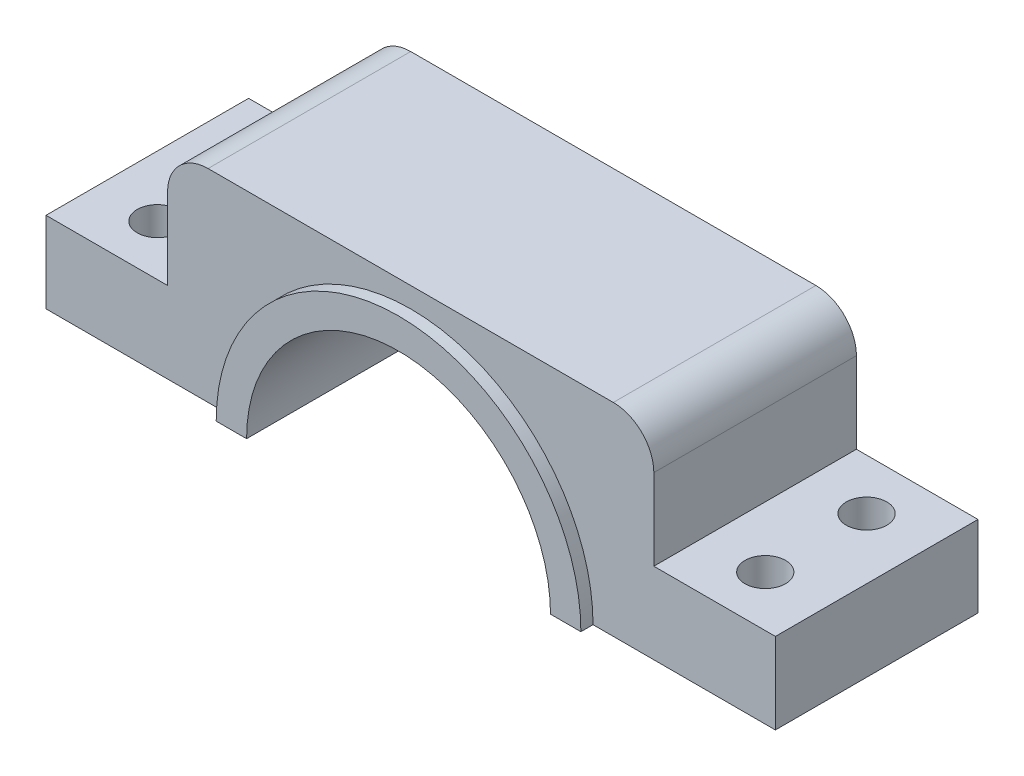
SolidWorks part; units mm, degrees
ref_plane "前视基准面" through (0, 0, 0) normal (0, 0, 1) x (1, 0, 0)
ref_plane "上视基准面" through (0, 0, 0) normal (0, 1, 0) x (1, 0, 0)
ref_plane "右视基准面" through (0, 0, 0) normal (1, 0, 0) x (0, 0, -1)
other "Configuration Table"
sketch "草图2" plane through (0, 0, 0) normal (0, 1, 0) x (1, 0, 0)
  line L1 (-60, -25) -> (60, -25)
  line L2 (-60, -25) -> (-60, 25)
  line L3 (-60, 25) -> (60, 25)
  line L4 (60, -25) -> (60, 25)
  line L5 (-60, -25) -> (60, 25) construction
  line L6 (-60, 25) -> (60, -25) construction
  point P0 (0, 0)
  dimension "D1" = 120
  dimension "D2" = 50
extrude "凸台-拉伸1" add sketch "草图2" along normal blind 50 contours L1 L4 L3 L2
sketch "草图3" plane through (0, 0, 25) normal (0, 0, 1) x (1, 0, 0)
  circle A0 centre (0, 0) radius 37.5
  dimension "D1" = 75
extrude "切除-拉伸1" cut sketch "草图3" against normal blind 139 contours A0
fillet "圆角1" radius 10 2 edges at (60, 50, 0) (-60, 50, 0)
sketch "草图4" plane through (0, 0, 0) normal (0, -1, 0) x (1, 0, 0)
  line L1 (-90, -25) -> (-60, -25)
  line L2 (-90, -25) -> (-90, 25)
  line L3 (-90, 25) -> (-60, 25)
  line L4 (90, -25) -> (90, 25)
  line L5 (-90, -25) -> (90, 25) construction
  line L6 (-90, 25) -> (90, -25) construction
  line L7 (37.5, 25) -> (60, 25) construction
  line L8 (60, 25) -> (60, -25) construction
  line L9 (-60, 25) -> (-60, -25) construction
  line L10 (60, 25) -> (60, -25)
  line L11 (-60, 25) -> (-60, -25)
  line L12 (60, 25) -> (90, 25)
  line L13 (60, -25) -> (90, -25)
  point P0 (0, 0)
  point P6 (0, 0)
  dimension "D1" = 180
extrude "凸台-拉伸2" add sketch "草图4" against normal blind 20
sketch "草图5" plane through (0, 0, 25) normal (0, 0, 1) x (1, 0, 0)
  line L0 (-45, 0) -> (-37.5, 0)
  line L3 (37.5, 0) -> (45, 0)
  arc A0 (37.5, 0) -> (-37.5, 0) centre (0, 0) ccw construction
  arc A1 (37.5, 0) -> (-37.5, 0) centre (0, 0) ccw
  arc A2 (45, 0) -> (-45, 0) centre (0, 0) ccw
  dimension "D1" = 90
extrude "凸台-拉伸3" add sketch "草图5" along normal blind 3
mirror "镜向1" about plane through (0, 0, 0) normal (0, 0, 1) of "凸台-拉伸3"
sketch "草图6" plane through (0, 20, 0) normal (0, 1, 0) x (1, 0, 0)
  line L0 (0, 0) -> (0, 41.2805) construction
  line L1 (-90, 25) -> (-60, 25) construction
  line L2 (-60, -25) -> (-90, -25) construction
  circle A0 centre (-75, 12.5) radius 5
  circle A1 centre (-75, -12.5) radius 5
  circle A2 centre (75, -12.5) radius 5
  circle A3 centre (75, 12.5) radius 5
  dimension "D4" = 10
  dimension "D1" = 75
  dimension "D2" = 12.5
  dimension "D3" = 12.5
extrude "切除-拉伸2" cut sketch "草图6" against normal blind 38
